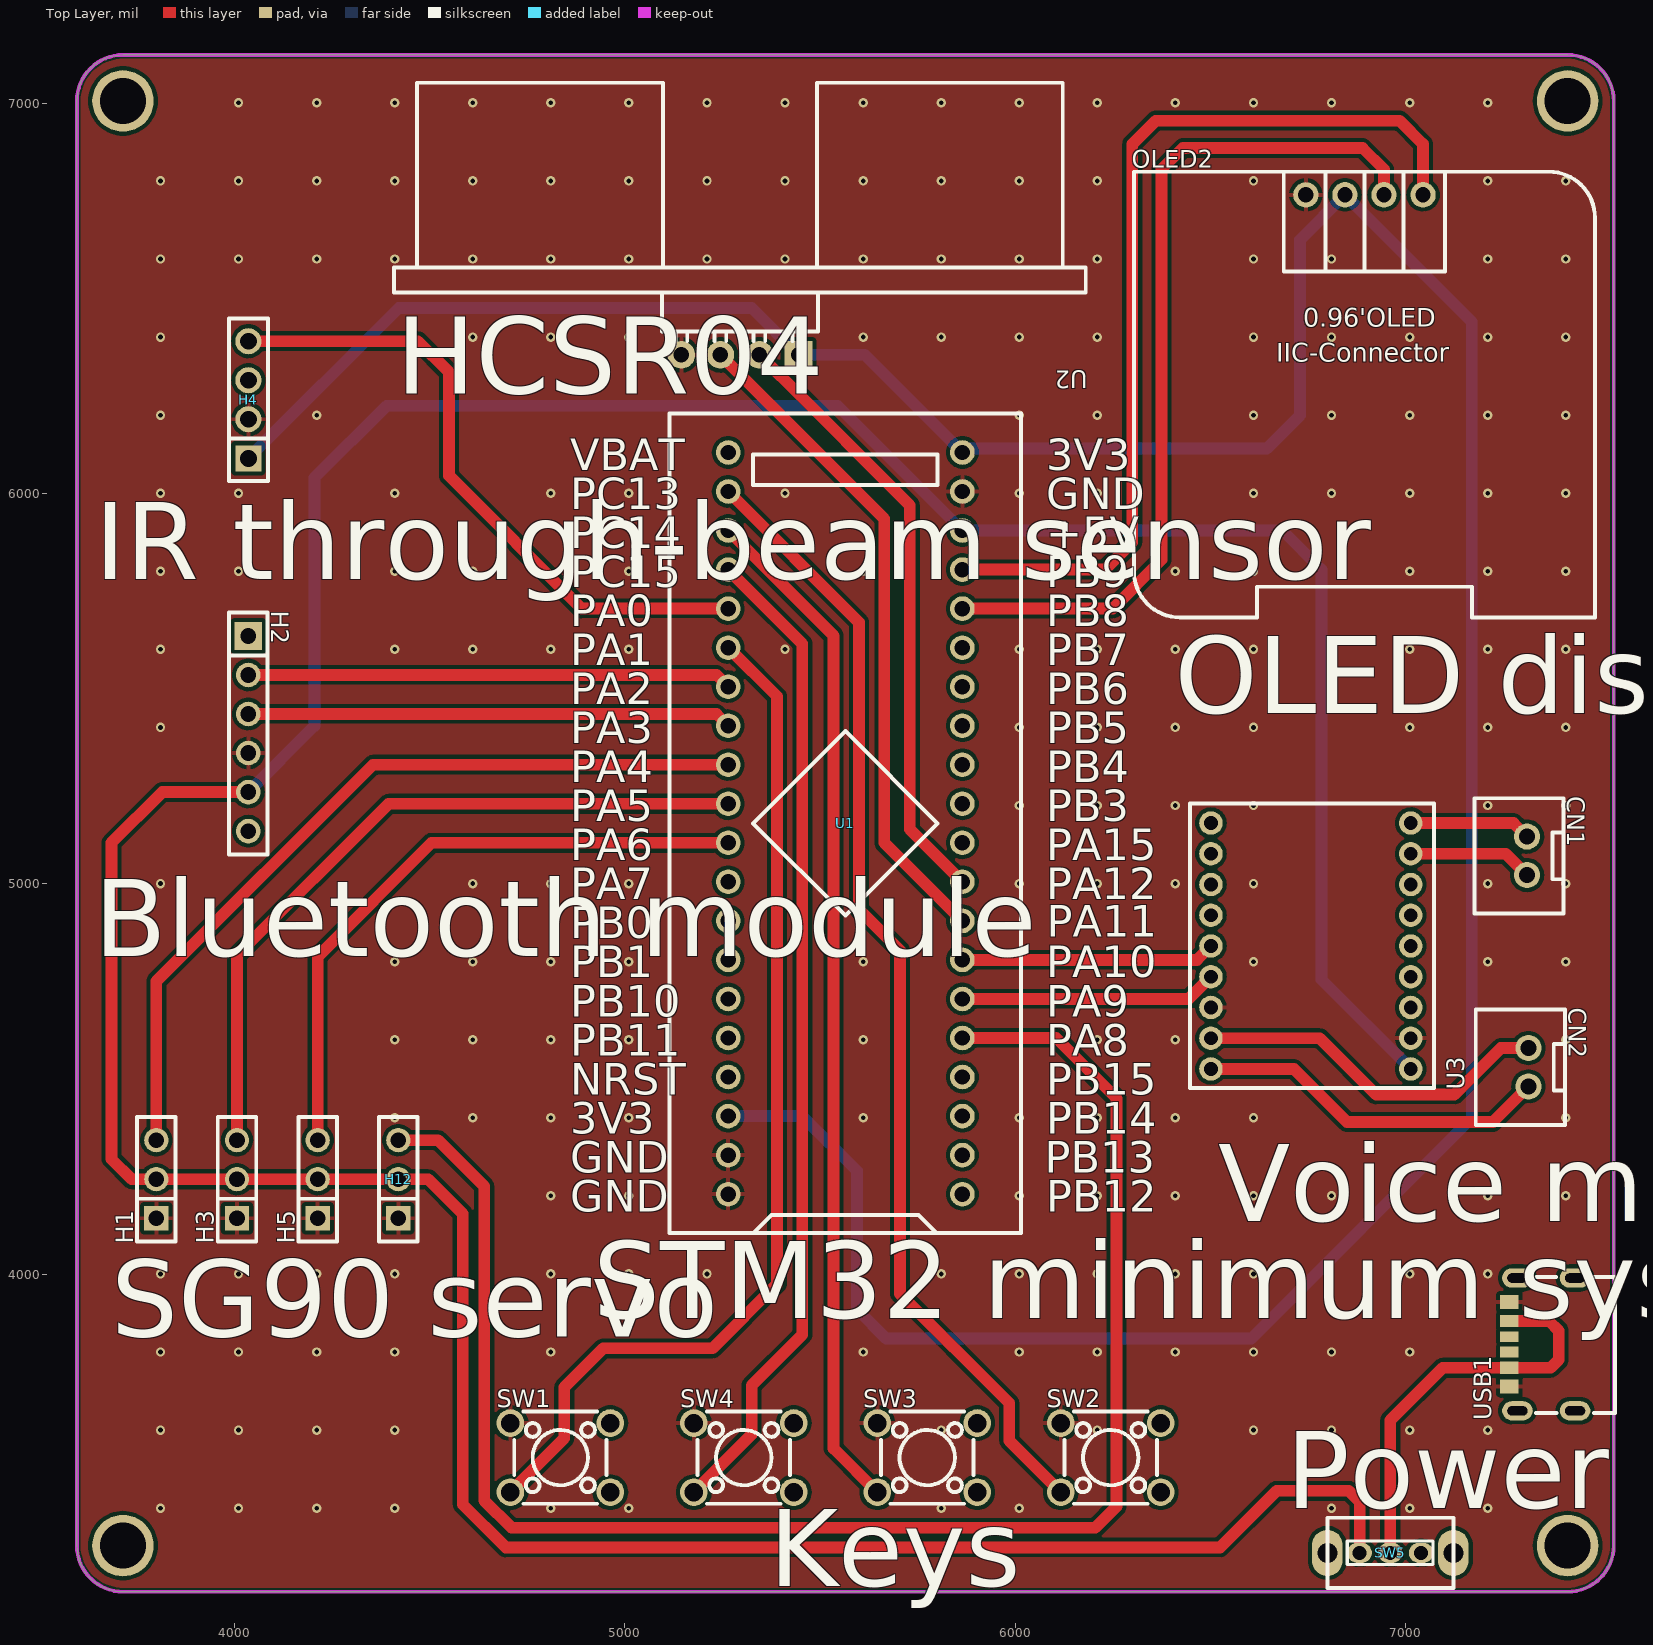
[diagram p0: Top Layer view]
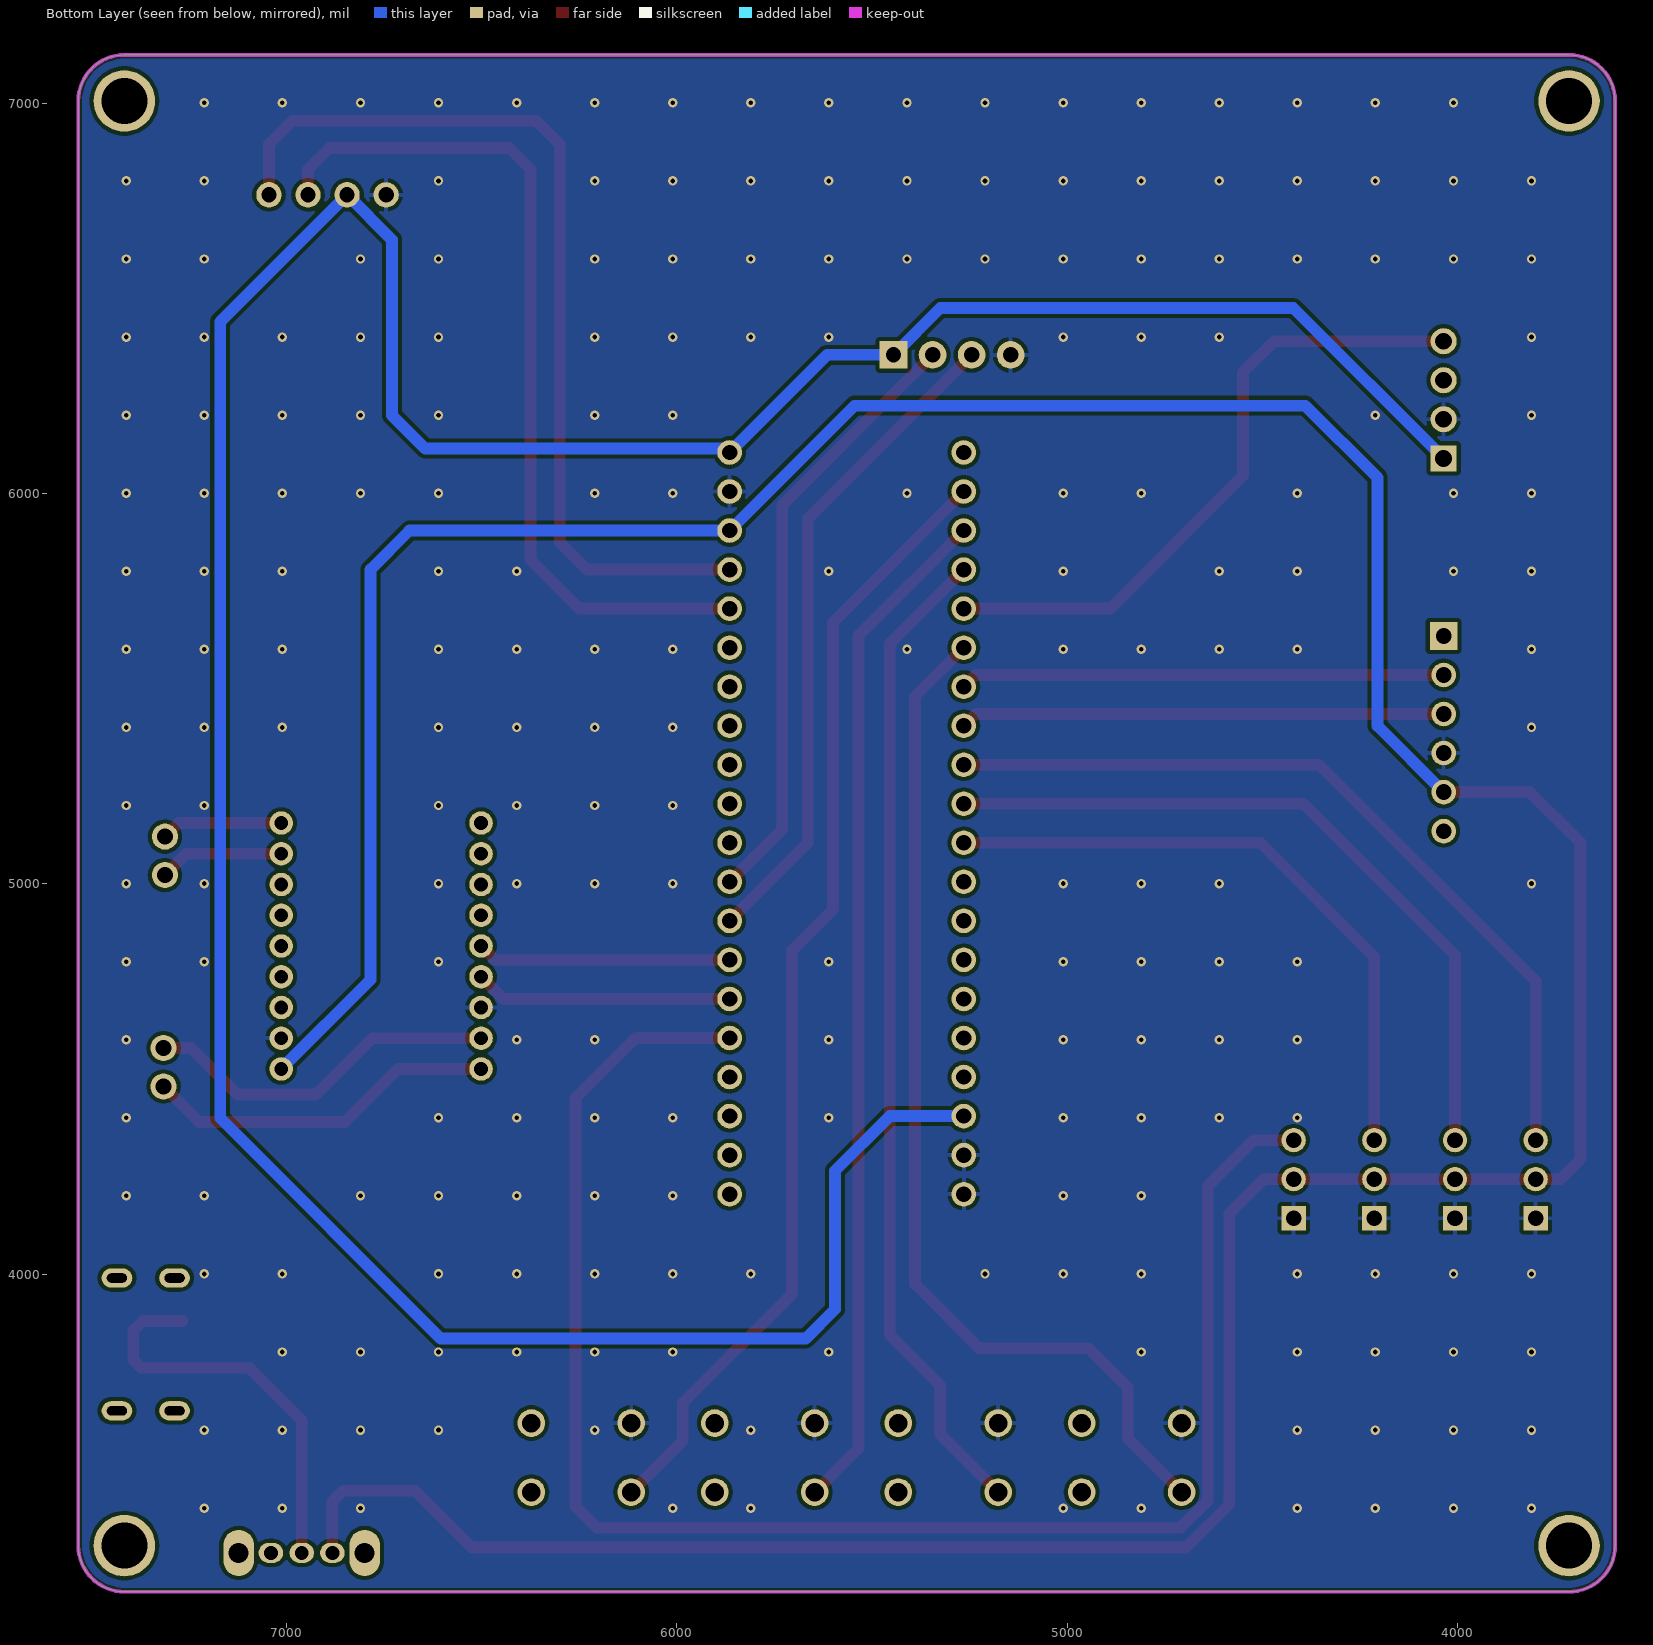
[diagram p1: Bottom Layer view, seen from below]
# Altium PCB MISC51947.pcbdoc
Units mil, origin at the board's own origin, x right, y up, seen from the top; angles counter-clockwise.
Board outline 3937.01 x 3937.01 mil, 2 copper layers (Top Layer, Bottom Layer), stack 62.206 mil thick; 18 components, 42 nets, 127 pads, 215 vias.

## Layer stack, top to bottom
Top Solder Mask Layer: solder mask 0.394, Dk 3.3
Top Layer: signal copper 1.379
Dielectric1: surface 59.449, FR4, Dk 4.5
Bottom Layer: signal copper 1.378
Bottom Solder Mask Layer: solder mask 0.394, Dk 3.3

## Board outline
3714.61,7123.5 ccw(c3714.61,7005.39) 3596.5,7005.39 3596.5,3304.61 ccw(c3714.61,3304.61) 3714.61,3186.5 7415.39,3186.5 ccw(c7415.39,3304.61) 7533.5,3304.61 7533.5,7005.39 ccw(c7415.39,7005.39) 7415.39,7123.5 3714.61,7123.5

## Design rules (kind name [scope] priority, off if disabled: settings)
BoardOutlineClearance copperThickness2oz_1 [All] p2 off: genericclearance=7.99 ignorepadtopadclearanceinfootprint=FALSE except(0: Arc-SplitContinuation Track-SplitContinuation SMDPad-SplitContinuation THPad-SplitContinuation Via-SplitContinuation Fill-SplitContinuation Region-SplitContinuation Poly-SplitContinuation Text-SplitContinuation Hole-SplitContinuation; 5.98: Arc-CutoutEdge Track-CutoutEdge SMDPad-CutoutEdge THPad-CutoutEdge Via-CutoutEdge Text-CutoutEdge; 6.9: Hole-OutlineEdge Hole-CutoutEdge; 10: Poly-OutlineEdge Poly-CutoutEdge; 11.81: Arc-OutlineEdge Track-OutlineEdge SMDPad-OutlineEdge THPad-OutlineEdge Via-OutlineEdge Fill-OutlineEdge Region-OutlineEdge Text-OutlineEdge Fill-CutoutEdge Region-CutoutEdge)
BoardOutlineClearance Plane_innerPlane_1 [All] p4 off: genericclearance=4.02 ignorepadtopadclearanceinfootprint=FALSE except(0: Arc-SplitContinuation Track-SplitContinuation SMDPad-SplitContinuation THPad-SplitContinuation Via-SplitContinuation Fill-SplitContinuation Region-SplitContinuation Poly-SplitContinuation Text-SplitContinuation Hole-SplitContinuation; 5.98: Arc-CutoutEdge Track-CutoutEdge SMDPad-CutoutEdge THPad-CutoutEdge Via-CutoutEdge Text-CutoutEdge; 6.9: Hole-OutlineEdge Hole-CutoutEdge; 10: Poly-OutlineEdge Poly-CutoutEdge; 11.81: Arc-OutlineEdge Track-OutlineEdge SMDPad-OutlineEdge THPad-OutlineEdge Via-OutlineEdge Fill-OutlineEdge Region-OutlineEdge Text-OutlineEdge Fill-CutoutEdge Region-CutoutEdge)
BoardOutlineClearance Copper_copperRegion_1 [All] p6 off: genericclearance=4.02 ignorepadtopadclearanceinfootprint=FALSE except(0: Arc-SplitContinuation Track-SplitContinuation SMDPad-SplitContinuation THPad-SplitContinuation Via-SplitContinuation Fill-SplitContinuation Region-SplitContinuation Poly-SplitContinuation Text-SplitContinuation Hole-SplitContinuation; 5.98: Arc-CutoutEdge Track-CutoutEdge SMDPad-CutoutEdge THPad-CutoutEdge Via-CutoutEdge Text-CutoutEdge; 6.9: Hole-OutlineEdge Hole-CutoutEdge; 10: Poly-OutlineEdge Poly-CutoutEdge; 11.81: Arc-OutlineEdge Track-OutlineEdge SMDPad-OutlineEdge THPad-OutlineEdge Via-OutlineEdge Fill-OutlineEdge Region-OutlineEdge Text-OutlineEdge Fill-CutoutEdge Region-CutoutEdge)
BoardOutlineClearance Copper_copperRegion_copperThickness1oz_1 [All] p8 off: genericclearance=4.02 ignorepadtopadclearanceinfootprint=FALSE except(0: Arc-SplitContinuation Track-SplitContinuation SMDPad-SplitContinuation THPad-SplitContinuation Via-SplitContinuation Fill-SplitContinuation Region-SplitContinuation Poly-SplitContinuation Text-SplitContinuation Hole-SplitContinuation; 5.98: Arc-CutoutEdge Track-CutoutEdge SMDPad-CutoutEdge THPad-CutoutEdge Via-CutoutEdge Text-CutoutEdge; 6.9: Hole-OutlineEdge Hole-CutoutEdge; 10: Poly-OutlineEdge Poly-CutoutEdge; 11.81: Arc-OutlineEdge Track-OutlineEdge SMDPad-OutlineEdge THPad-OutlineEdge Via-OutlineEdge Fill-OutlineEdge Region-OutlineEdge Text-OutlineEdge Fill-CutoutEdge Region-CutoutEdge)
BoardOutlineClearance Copper_copperRegion_Copper_copperRegion_1 [All] p10 off: genericclearance=4.02 ignorepadtopadclearanceinfootprint=FALSE except(0: Arc-SplitContinuation Track-SplitContinuation SMDPad-SplitContinuation THPad-SplitContinuation Via-SplitContinuation Fill-SplitContinuation Region-SplitContinuation Poly-SplitContinuation Text-SplitContinuation Hole-SplitContinuation; 5.98: Arc-CutoutEdge Track-CutoutEdge SMDPad-CutoutEdge THPad-CutoutEdge Via-CutoutEdge Text-CutoutEdge; 6.9: Hole-OutlineEdge Hole-CutoutEdge; 10: Poly-OutlineEdge Poly-CutoutEdge; 11.81: Arc-OutlineEdge Track-OutlineEdge SMDPad-OutlineEdge THPad-OutlineEdge Via-OutlineEdge Fill-OutlineEdge Region-OutlineEdge Text-OutlineEdge Fill-CutoutEdge Region-CutoutEdge)
BoardOutlineClearance copperThickness1oz_1 [All] p12: genericclearance=4.02 ignorepadtopadclearanceinfootprint=FALSE except(0: Arc-SplitContinuation Track-SplitContinuation SMDPad-SplitContinuation THPad-SplitContinuation Via-SplitContinuation Fill-SplitContinuation Region-SplitContinuation Poly-SplitContinuation Text-SplitContinuation Hole-SplitContinuation; 5.98: Arc-CutoutEdge Track-CutoutEdge SMDPad-CutoutEdge THPad-CutoutEdge Via-CutoutEdge Text-CutoutEdge; 6.9: Hole-OutlineEdge Hole-CutoutEdge; 10: Poly-OutlineEdge Poly-CutoutEdge; 11.81: Arc-OutlineEdge Track-OutlineEdge SMDPad-OutlineEdge THPad-OutlineEdge Via-OutlineEdge Fill-OutlineEdge Region-OutlineEdge Text-OutlineEdge Fill-CutoutEdge Region-CutoutEdge)
Clearance copperThickness2oz [All] p1 off: gap=7.99 ignorepadtopadclearanceinfootprint=FALSE except(5.98: SMDPad-Track SMDPad-SMDPad THPad-Track SMDPad-THPad THPad-THPad Track-Via SMDPad-Via THPad-Via Via-Via Fill-SMDPad Region-SMDPad Fill-THPad Region-THPad Fill-Via Region-Via Fill-Fill Fill-Region Region-Region Arc-Track Arc-SMDPad Arc-THPad Arc-Via Fill-Arc Region-Arc Arc-Arc Text-Track SMDPad-Text Text-THPad Text-Via Fill-Text Region-Text Arc-Text Text-Text; 6.9: Hole-Track Hole-SMDPad Hole-THPad Hole-Via Fill-Hole Region-Hole Hole-Arc Hole-Text; 10: Poly-Track Poly-SMDPad Poly-THPad Poly-Via Poly-Fill Poly-Region Poly-Poly Poly-Arc Poly-Text Poly-Hole; 11.81: Fill-Track Region-Track)
Clearance Plane_innerPlane [All] p3 off: gap=4.02 ignorepadtopadclearanceinfootprint=FALSE except(5.98: SMDPad-Track SMDPad-SMDPad THPad-Track SMDPad-THPad THPad-THPad Track-Via SMDPad-Via THPad-Via Via-Via Fill-SMDPad Region-SMDPad Fill-THPad Region-THPad Fill-Via Region-Via Fill-Fill Fill-Region Region-Region Arc-Track Arc-SMDPad Arc-THPad Arc-Via Fill-Arc Region-Arc Arc-Arc Text-Track SMDPad-Text Text-THPad Text-Via Fill-Text Region-Text Arc-Text Text-Text; 6.9: Hole-Track Hole-SMDPad Hole-THPad Hole-Via Fill-Hole Region-Hole Hole-Arc Hole-Text; 10: Poly-Track Poly-SMDPad Poly-THPad Poly-Via Poly-Fill Poly-Region Poly-Poly Poly-Arc Poly-Text Poly-Hole; 11.81: Fill-Track Region-Track)
Clearance Copper_copperRegion [All] p5 off: gap=4.02 ignorepadtopadclearanceinfootprint=FALSE except(5.98: SMDPad-Track SMDPad-SMDPad THPad-Track SMDPad-THPad THPad-THPad Track-Via SMDPad-Via THPad-Via Via-Via Fill-SMDPad Region-SMDPad Fill-THPad Region-THPad Fill-Via Region-Via Fill-Fill Fill-Region Region-Region Arc-Track Arc-SMDPad Arc-THPad Arc-Via Fill-Arc Region-Arc Arc-Arc Text-Track SMDPad-Text Text-THPad Text-Via Fill-Text Region-Text Arc-Text Text-Text; 6.9: Hole-Track Hole-SMDPad Hole-THPad Hole-Via Fill-Hole Region-Hole Hole-Arc Hole-Text; 10: Poly-Track Poly-SMDPad Poly-THPad Poly-Via Poly-Fill Poly-Region Poly-Poly Poly-Arc Poly-Text Poly-Hole; 11.81: Fill-Track Region-Track)
Clearance Copper_copperRegion_copperThickness1oz [All] p7 off: gap=4.02 ignorepadtopadclearanceinfootprint=FALSE except(5.98: SMDPad-Track SMDPad-SMDPad THPad-Track SMDPad-THPad THPad-THPad Track-Via SMDPad-Via THPad-Via Via-Via Fill-SMDPad Region-SMDPad Fill-THPad Region-THPad Fill-Via Region-Via Fill-Fill Fill-Region Region-Region Arc-Track Arc-SMDPad Arc-THPad Arc-Via Fill-Arc Region-Arc Arc-Arc Text-Track SMDPad-Text Text-THPad Text-Via Fill-Text Region-Text Arc-Text Text-Text; 6.9: Hole-Track Hole-SMDPad Hole-THPad Hole-Via Fill-Hole Region-Hole Hole-Arc Hole-Text; 10: Poly-Track Poly-SMDPad Poly-THPad Poly-Via Poly-Fill Poly-Region Poly-Poly Poly-Arc Poly-Text Poly-Hole; 11.81: Fill-Track Region-Track)
Clearance Copper_copperRegion_Copper_copperRegion [All] p9 off: gap=4.02 ignorepadtopadclearanceinfootprint=FALSE except(5.98: SMDPad-Track SMDPad-SMDPad THPad-Track SMDPad-THPad THPad-THPad Track-Via SMDPad-Via THPad-Via Via-Via Fill-SMDPad Region-SMDPad Fill-THPad Region-THPad Fill-Via Region-Via Fill-Fill Fill-Region Region-Region Arc-Track Arc-SMDPad Arc-THPad Arc-Via Fill-Arc Region-Arc Arc-Arc Text-Track SMDPad-Text Text-THPad Text-Via Fill-Text Region-Text Arc-Text Text-Text; 6.9: Hole-Track Hole-SMDPad Hole-THPad Hole-Via Fill-Hole Region-Hole Hole-Arc Hole-Text; 10: Poly-Track Poly-SMDPad Poly-THPad Poly-Via Poly-Fill Poly-Region Poly-Poly Poly-Arc Poly-Text Poly-Hole; 11.81: Fill-Track Region-Track)
Clearance copperThickness1oz [All] p11: gap=4.02 ignorepadtopadclearanceinfootprint=FALSE except(5.98: SMDPad-Track SMDPad-SMDPad THPad-Track SMDPad-THPad THPad-THPad Track-Via SMDPad-Via THPad-Via Via-Via Fill-SMDPad Region-SMDPad Fill-THPad Region-THPad Fill-Via Region-Via Fill-Fill Fill-Region Region-Region Arc-Track Arc-SMDPad Arc-THPad Arc-Via Fill-Arc Region-Arc Arc-Arc Text-Track SMDPad-Text Text-THPad Text-Via Fill-Text Region-Text Arc-Text Text-Text; 6.9: Hole-Track Hole-SMDPad Hole-THPad Hole-Via Fill-Hole Region-Hole Hole-Arc Hole-Text; 10: Poly-Track Poly-SMDPad Poly-THPad Poly-Via Poly-Fill Poly-Region Poly-Poly Poly-Arc Poly-Text Poly-Hole; 11.81: Fill-Track Region-Track)
DiffPairsRouting differentialPair [All] p1: maxlimit=6 minlimit=6 mostfreqgap=6 toplayer_minwidth=5 toplayer_prefwidth=10 toplayer_maxwidth=100 toplayer_mingap=6 toplayer_prefgap=6 toplayer_maxgap=6 bottomlayer_minwidth=5 bottomlayer_prefwidth=10 bottomlayer_maxwidth=100 bottomlayer_mingap=6 bottomlayer_prefgap=6 bottomlayer_maxgap=6 maxuncoupledlength=10
HoleToHoleClearance otherClearance [All] p1: gap=11.81 allowstackedmicrovias=TRUE
Length netLength [All] p1: minlimit=0 maxlimit=0
PasteMaskExpansion pasteMaskExpansion [All] p1: expansion=0
PlaneConnect innerPlane [All] p1: planeconnectstyle=Relief reliefexpansion=20 reliefentries=4 reliefconductorwidth=10 reliefairgap=10
PolygonConnect copperRegion_copperThickness1oz [All] p1 off: connectstyle=Relief reliefconductorwidth=10 reliefentries=4 polygonreliefangle="90 Angle" airgapwidth=10 via.connectstyle=Relief via.reliefconductorwidth=10 via.reliefentries=4 via.polygonreliefangle="90 Angle" via.airgapwidth=10
PolygonConnect copperRegion_Copper_copperRegion [All] p2 off: connectstyle=Relief reliefconductorwidth=10 reliefentries=4 polygonreliefangle="90 Angle" airgapwidth=10 via.connectstyle=Relief via.reliefconductorwidth=10 via.reliefentries=4 via.polygonreliefangle="90 Angle" via.airgapwidth=10
PolygonConnect copperRegion [All] p3: connectstyle=Relief reliefconductorwidth=10 reliefentries=4 polygonreliefangle="90 Angle" airgapwidth=10 via.connectstyle=Relief via.reliefconductorwidth=10 via.reliefentries=4 via.polygonreliefangle="90 Angle" via.airgapwidth=10
RoutingVias viaSize [All] p1: holewidth=12.01 width=24.02 viastyle="Through Hole" minholewidth=11.81 minwidth=19.68 maxholewidth=248.03 maxwidth=393.7
SolderMaskExpansion solderMaskExpansion [IsVia] p1: expansion=-1000 istentingtop=TRUE
SolderMaskExpansion solderMaskExpansion [All] p2: expansion=2 istentingtop=FALSE
Width copperThickness2oz_2 [All] p1 off: maxlimit=100 minlimit=8 preferedwidth=10
Width copperThickness1oz_2 [All] p2: maxlimit=100 minlimit=5 preferedwidth=10

## Components (designator, comment, footprint, x,y, rotation, side; value= is the part's Value field where it differs from the comment)
CN1 "XH2.54*2P_THT" CONN-TH_2P-P2.50-XH2.54-2P 7311.56,5071.57 r270 top
CN2 "XH2.54*2P_THT" CONN-TH_2P-P2.50-XH2.54-2P 7315,4530 r270 top
H1 "" HDR-TH_3P-P2.54-V-F 3800,4243.21 r90 top
H2 "" HDR-TH_6P-P2.54-V-F 4035.79,5385 r270 top
H3 "" HDR-TH_3P-P2.54-V-F 4006.67,4243.21 r90 top
H4 "" HDR-TH_4P-P2.54-V-F 4035.79,6240 r90 top
H5 "" HDR-TH_3P-P2.54-V-F 4213.33,4243.21 r90 top
H12 "" HDR-TH_3P-P2.54-V-F 4420,4243.21 r90 top
OLED2 "" 0.96OLED_4P 6895,6765 r0 top
SW1 "" SW-TH_4P-L6.0-W6.0-P4.50-LS6.5 4835,3530 r0 top
SW2 "" SW-TH_4P-L6.0-W6.0-P4.50-LS6.5 6245,3530 r0 top
SW3 "" SW-TH_4P-L6.0-W6.0-P4.50-LS6.5 5775,3530 r0 top
SW4 "" SW-TH_4P-L6.0-W6.0-P4.50-LS6.5 5305,3530 r0 top
SW5 "" 拨动开关 6956,3286 r0 top
U1 "STM32F103C8T6-Card" CONN-TH_L53.3-W22.9_STM32F103C8T6-CARD 5565,5155 r90 top
U2 "HC-SR04" TH_HC-SR04V 5295,6355 r180 top
U3 "CON2.0MM-PAD-18" CONN-TH_18P-P2.00_C9900078766 7013.53,4840.71 r90 top
USB1 "" "USB_ TYPE-C-6P" 7350.24,3815.09 r90 top

## Footprints (in the part's own frame and the unit in brackets; to place one, negate y for a bottom-side part, rotate by r counter-clockwise, add the part's x,y. Pads: shape width x height; smd on the part's side, far side on the other; paste and mask are expansions set on the pad)
0.96OLED_4P [mm]
  round 1.65 hole 1 copper offset 0,0: 1(-3.81,-0.001) 2(-1.27,0.002) 3(1.27,0.002) 4(3.81,0.002)
  silkscreen extent -15,-27.5 15,1.5
CONN-TH_2P-P2.50-XH2.54-2P [mm]
  round 1.7 hole 1.05 paste+0 mask+0.05: 1(1.25,0) 2(-1.25,0)
  silkscreen extent -3.75,-3.42 3.75,2.37
CONN-TH_18P-P2.00_C9900078766 [mil]
  round 60 hole 35.43 paste+0 mask+1.97: 1(-314.96,0.01) 2(-314.96,511.81) 3(-236.22,0.01) 4(-236.22,511.81) 5(-157.48,0.01) 6(-157.48,511.81) 9(0,0) 10(0,511.81) 11(78.74,0) 12(78.74,511.81) 13(157.48,0) 14(157.48,511.81) 15(236.22,0) 16(236.22,511.81) 17(314.96,0) 18(314.96,511.81)
  round 60 hole 35.43 copper offset -0.01,0 paste+0 mask+1.97: 7(-78.72,0.01) 8(-78.72,511.81)
  silkscreen extent -363,-60 365,565
CONN-TH_L53.3-W22.9_STM32F103C8T6-CARD [mm]
  round 1.6 hole 1: 1(-24.13,-7.62) 2(-21.59,-7.62) 3(-19.05,-7.62) 4(-16.51,-7.62) 5(-13.97,-7.62) 6(-11.43,-7.62) 7(-8.89,-7.62) 8(-6.35,-7.62) 9(-3.81,-7.62) 10(-1.27,-7.62) 11(1.27,-7.62) 12(3.81,-7.62) 13(6.35,-7.62) 14(8.89,-7.62) 15(11.43,-7.62) 16(13.97,-7.62) 17(16.51,-7.62) 18(19.05,-7.62) 19(21.59,-7.62) 20(24.13,-7.62) 21(24.13,7.62) 22(21.59,7.62) 23(19.05,7.62) 24(16.51,7.62) 25(13.97,7.62) 26(11.43,7.62) 27(8.89,7.62) 28(6.35,7.62) 29(3.81,7.62) 30(1.27,7.62) 31(-1.27,7.62) 32(-3.81,7.62) 33(-6.35,7.62) 34(-8.89,7.62) 35(-11.43,7.62) 36(-13.97,7.62) 37(-16.51,7.62) 38(-19.05,7.62) 39(-21.59,7.62) 40(-24.13,7.62)
  silkscreen extent -26.67,-11.43 26.67,11.43
HDR-TH_3P-P2.54-V-F [mil]
  rect 62x62 hole 40.16: 1(-100,0)
  round 62 hole 40.16: 2(0,0) 3(100,0)
  silkscreen extent -160,-49 160,49
HDR-TH_4P-P2.54-V-F [mm]
  rect 1.7x1.7 hole 1.1: 1(-3.81,0)
  round 1.7 hole 1.1: 2(-1.27,0) 3(1.27,0) 4(3.81,0)
  silkscreen extent -5.29,-1.27 5.29,1.27
HDR-TH_6P-P2.54-V-F [mm]
  rect 1.8x1.8 hole 1.02: 1(-6.35,0)
  round 1.6 hole 1.02: 2(-3.81,0) 3(-1.27,0) 4(1.27,0) 5(3.81,0) 6(6.35,0)
  silkscreen extent -7.87,-1.25 7.87,1.25
SW-TH_4P-L6.0-W6.0-P4.50-LS6.5 [mm]
  round 1.8 hole 1.2: 1(-3.25,2.25) 2(3.25,2.25) 3(-3.25,-2.25) 4(3.25,-2.25)
  silkscreen extent -3,-3 3,3
TH_HC-SR04V [mm]
  rect 1.8x1.8 hole 1.001: 1(-3.81,0)
  round 1.8 hole 1.001: 2(-1.27,0) 3(1.27,0) 4(3.81,0)
  silkscreen extent -22.5,-17.7 22.5,-0.89
"USB_ TYPE-C-6P" [mm]
  oval 1.25x2 hole 0.6 slot 1.3 at 90 deg paste+0 mask+0.05: 7(-4.193,1.611) 8(4.447,1.611) 9(-4.193,-2.139) 10(4.447,-2.139)
  rect 0.7x1.2 smd paste-100 mask+0.05: A5(-0.373,2.139) B5(0.627,2.139)
  rect 0.8x1.2 smd paste-100 mask+0.05: A9(1.647,2.139) B9(-1.393,2.139)
  rect 0.9x1.2 smd paste-100 mask+0.05: A12(2.877,2.139) B12(-2.623,2.139)
  silkscreen extent -4.34,-4.75 4.52,0.39
拨动开关 [mil]
  oval 63x51.2 hole 35.4 paste+0 mask+2: 1(-73.4,0) 2(5,0) 3(84,0)
  oval 78.7x118.1 hole 51.2 paste+0 mask+2: 4(166.7,0) 5(-156.1,0)
  silkscreen extent -156,-90 167,90

## Free pads (board coordinates)
  round 157.48 hole 118.11: 1(3714.61,7005.39) 1(3714.61,3304.61) 1(7415.39,7005.39) 1(7415.39,3304.61)

## Via types
v1: diameter 24.02, hole 12, Top Layer to Bottom Layer, 215 vias

## Nets (pads, with @x,y where several pads share a name; then routed paths per layer and width w, separated by ;. In a path a pad name is that pad's centre, name@x,y a point inside that pad or via, vN(x,y) a via of type N, cw(c..) or ccw(c..) an arc to the next point about the centre after c; other vN are vias at no path point)
$1N17172: SW5.2 USB1.A9 USB1.B9 | length 1046.6
  Top Layer w30: SW5.2 6961,3626 7095.25,3760.25 USB1.B9 7371.97,3760.25 7392.43,3780.7 7392.43,3855.17 7367.68,3879.93 USB1.A9
+5V: H1.2 H2.5 H3.2 H5.2 H12.2 SW5.1 U1.18 U3.1 | length 10543.3
  Top Layer w30: H2.5 3815,5235 3685,5105 3685,4295 3736.79,4243.21 H1.2 H3.2 H5.2 H12.2 4496.79,4243.21 4585,4155 4585,3410 4695,3300 6525,3300 6670,3445 6855,3445 6882.6,3417.4 SW5.1
  Bottom Layer w30: H2.5 4205,5404.21 4205,6040 4390,6225 5545,6225 U1.18 6685,5905 6785,5805 6785,4754.27 U3.1
GND: H1.1 H2.4 H3.1 H4.2 H5.1 H12.1 OLED2.1 SW1.1 SW2.1 SW3.1 SW4.1 U1.19 U1.39 U1.40 U2.4 U3.3 U3.6 USB1.A12 USB1.B12
  other v1: 3810.6,3400.6 4010.6,3400.6 4210.6,3400.6 4410.6,3400.6 4810.6,3400.6 5010.6,3400.6 5810.6,3400.6 6010.6,3400.6 6810.6,3400.6 7010.6,3400.6 7210.6,3400.6 3810.6,3600.6 4010.6,3600.6 4210.6,3600.6 4410.6,3600.6 5810.6,3600.6 6210.6,3600.6 6610.6,3600.6 6810.6,3600.6 7010.6,3600.6 7210.6,3600.6 3810.6,3800.6 4010.6,3800.6 4210.6,3800.6 4410.6,3800.6 4810.6,3800.6 5610.6,3800.6 6010.6,3800.6 6210.6,3800.6 6410.6,3800.6 6610.6,3800.6 6810.6,3800.6 7010.6,3800.6 3810.6,4000.6 4010.6,4000.6 4210.6,4000.6 4410.6,4000.6 4810.6,4000.6 5010.6,4000.6 5210.6,4000.6 5810.6,4000.6 6010.6,4000.6 6210.6,4000.6 6410.6,4000.6 6610.6,4000.6 7010.6,4000.6 7210.6,4000.6 4810.6,4200.6 5010.6,4200.6 6010.6,4200.6 6210.6,4200.6 6410.6,4200.6 6610.6,4200.6 6810.6,4200.6 7210.6,4200.6 7410.6,4200.6 4410.6,4400.6 4610.6,4400.6 4810.6,4400.6 5010.6,4400.6 5610.6,4400.6 6010.6,4400.6 6210.6,4400.6 6410.6,4400.6 6610.6,4400.6 7410.6,4400.6 4410.6,4600.6 4610.6,4600.6 4810.6,4600.6 5010.6,4600.6 5610.6,4600.6 6210.6,4600.6 6410.6,4600.6 7410.6,4600.6 4410.6,4800.6 4610.6,4800.6 4810.6,4800.6 5010.6,4800.6 5610.6,4800.6 6610.6,4800.6 7210.6,4800.6 7410.6,4800.6 3810.6,5000.6 4610.6,5000.6 4810.6,5000.6 5010.6,5000.6 6010.6,5000.6 6210.6,5000.6 6410.6,5000.6 6610.6,5000.6 7210.6,5000.6 7410.6,5000.6 6010.6,5200.6 6210.6,5200.6 6410.6,5200.6 6610.6,5200.6 7210.6,5200.6 7410.6,5200.6 3810.6,5400.6 6010.6,5400.6 6210.6,5400.6 6410.6,5400.6 6610.6,5400.6 7010.6,5400.6 7210.6,5400.6 7410.6,5400.6 3810.6,5600.6 4410.6,5600.6 4610.6,5600.6 4810.6,5600.6 5010.6,5600.6 5410.6,5600.6 6010.6,5600.6 6210.6,5600.6 6410.6,5600.6 6610.6,5600.6 7010.6,5600.6 7210.6,5600.6 7410.6,5600.6 3810.6,5800.6 4010.6,5800.6 4410.6,5800.6 4610.6,5800.6 5010.6,5800.6 5610.6,5800.6 6410.6,5800.6 6610.6,5800.6 7010.6,5800.6 7210.6,5800.6 7410.6,5800.6 3810.6,6000.6 4010.6,6000.6 4410.6,6000.6 4810.6,6000.6 5010.6,6000.6 5410.6,6000.6 6010.6,6000.6 6210.6,6000.6 6610.6,6000.6 6810.6,6000.6 7010.6,6000.6 7210.6,6000.6 7410.6,6000.6 3810.6,6200.6 4210.6,6200.6 6010.6,6200.6 6210.6,6200.6 6610.6,6200.6 6810.6,6200.6 7010.6,6200.6 7210.6,6200.6 7410.6,6200.6 3810.6,6400.6 4610.6,6400.6 4810.6,6400.6 5010.6,6400.6 5610.6,6400.6 5810.6,6400.6 6010.6,6400.6 6210.6,6400.6 6610.6,6400.6 6810.6,6400.6 7010.6,6400.6 7210.6,6400.6 7410.6,6400.6 3810.6,6600.6 4010.6,6600.6 4210.6,6600.6 4410.6,6600.6 4610.6,6600.6 4810.6,6600.6 5010.6,6600.6 5210.6,6600.6 5410.6,6600.6 5610.6,6600.6 5810.6,6600.6 6010.6,6600.6 6210.6,6600.6 6610.6,6600.6 6810.6,6600.6 7210.6,6600.6 7410.6,6600.6 3810.6,6800.6 4010.6,6800.6 4210.6,6800.6 4410.6,6800.6 4610.6,6800.6 4810.6,6800.6 5010.6,6800.6 5210.6,6800.6 5410.6,6800.6 5610.6,6800.6 5810.6,6800.6 6010.6,6800.6 6210.6,6800.6 6610.6,6800.6 7210.6,6800.6 7410.6,6800.6 4010.6,7000.6 4210.6,7000.6 4410.6,7000.6 4610.6,7000.6 4810.6,7000.6 5010.6,7000.6 5210.6,7000.6 5410.6,7000.6 5610.6,7000.6 5810.6,7000.6 6010.6,7000.6 6210.6,7000.6 6410.6,7000.6 6610.6,7000.6 6810.6,7000.6 7010.6,7000.6 7210.6,7000.6
MIC+: CN1.1 U3.15 | length 320.6
  Top Layer w30: U3.15 7256.99,5076.93 CN1.1
MIC-: CN1.2 U3.17 | length 312.5
  Top Layer w30: U3.17 7276.68,5155.67 CN1.2
NRST: U1.37
PA0: H4.4 U1.25 | length 1668.2
  Top Layer w30: H4.4 4470,6390 4550,6310 4550,6045 4890,5705 U1.25
PA1: SW1.3 U1.26 | length 2662.3
  Top Layer w30: SW1.3 4845,3579.37 4845,3710 4945,3810 5225,3810 5390,3975 5390,5480 U1.26
PA2: H2.2 U1.27 | length 1241.6
  Top Layer w30: H2.2 5235,5535 U1.27
PA3: H2.3 U1.28 | length 1241.6
  Top Layer w30: H2.3 5235,5435 U1.28
PA4: H1.3 U1.29 | length 2101.7
  Top Layer w30: H1.3 3800,4750 4355,5305 U1.29
PA5: H3.3 U1.30 | length 1892.6
  Top Layer w30: H3.3 4006.67,4816.67 4395,5205 U1.30
PA6: H5.3 U1.31 | length 1642.6
  Top Layer w30: H5.3 4213.33,4813.33 4505,5105 U1.31
PA7: U1.32
PA8: H12.3 U1.5 | length 4249.9
  Top Layer w30: H12.3 4521.79,4343.21 4640,4225 4640,3420 4710,3350 6205,3350 6260,3405 6260,4450 6105,4605 U1.5
PA9: U1.6 U3.8 | length 660.3
  Top Layer w30: U1.6 6444.75,4705 U3.8
PA10: U1.7 U3.10 | length 651.5
  Top Layer w30: U1.7 6466.02,4805 U3.10
PA11: U1.8 U2.3 | length 1706.8
  Top Layer w30: U2.3 5665,5935 5665,5105 U1.8
PA12: U1.9 U2.2 | length 1565.4
  Top Layer w30: U2.2 5392.18,6307.82 ccw(c5409.57,6319.57) 5397.82,6302.18 5730,5970 5730,5140 U1.9
PA15: U1.10
PB0: U1.33
PB1: U1.34
PB3: U1.11
PB4: U1.12
PB5: U1.13
PB6: U1.14
PB7: U1.15
PB8: OLED2.3 U1.16 | length 2242.3
  Top Layer w30: U1.16 6250,5705 6375,5830 6375,6830 6430,6885 6890,6885 6945,6830 OLED2.3@6945,6765.05
PB9: OLED2.4 U1.17 | length 2408.7
  Top Layer w30: U1.17 6230,5805 6300,5875 6300,6895 6360,6955 6985,6955 7045,6895 OLED2.4@7045,6765.05
PB10: U1.35
PB11: U1.36
PB12: U1.1
PB13: U1.2
PB14: U1.3
PB15: U1.4
PC13: SW2.3 U1.22 | length 2916.5
  Top Layer w30: U1.22 5600,5670 5600,4935 5705,4830 5705,3950 5985,3670 5985,3573.47 SW2.3
PC14: SW3.3 U1.23 | length 2621.8
  Top Layer w30: U1.23 5535,5635 5535,3553.47 SW3.3
PC15: SW4.3 U1.24 | length 2557.4
  Top Layer w30: SW4.3 5325,3589.37 5325,3715 5455,3845 5455,5615 U1.24
SPK+: CN2.1 U3.2 | length 907.1
  Top Layer w30: U3.2 6714.25,4525.75 6850,4390 7224.22,4390 CN2.1
SPK-: CN2.2 U3.4 | length 922.5
  Top Layer w30: U3.4 6780.51,4604.49 6925,4460 7125,4460 7244.22,4579.22 CN2.2
VBAT: U1.21
VCC: H4.1 OLED2.2 U1.20 U1.38 U2.1 | length 8741.7
  Bottom Layer w30: H4.1 4420.79,6475 5325,6475 U2.1 5615,6355 U1.20 5875,6115 6645,6115 6730,6200 6730,6650.05 6845,6765.05 7170,6440.05 7170,4400 6605,3835 5670,3835 5595,3910 5595,4265 5455,4405 U1.38
pads on no net: H2.1 H2.6 H4.3 SW1.2 SW1.4 SW2.2 SW2.4 SW3.2 SW3.4 SW4.2 SW4.4 SW5.3 SW5.4 SW5.5 U3.5 U3.7 U3.9 U3.11 U3.12 U3.13 U3.14 U3.16 U3.18 USB1.7 USB1.8 USB1.9 USB1.10 USB1.A5 USB1.B5

## Polygon pours and split planes (outlines as drawn)
GND on Bottom Layer (solid, remove dead copper, pour order 2): 3525,7245 3525,3080 7700,3080 7700,7245
GND on Top Layer (solid, remove dead copper, pour order 2): 3000,7415 3000,3000 7930,3000 7930,7415

## Keep-outs
Board Outline Layer:
  the board outline again, w10

## Silkscreen, mask and mechanical layers (free items; w line width, h text height)
Top Silkscreen Layer:
  text "HCSR04" at 4415,6255 h196.85
  text "VBAT" at 4860.95,6060 h80
  text "3V3" at 6079.16,6060 h80
  text "PC13" at 4860.95,5960 h80
  text "GND" at 6079.16,5960 h80
  text "PC14" at 4860.95,5860 h80
  text "+5V" at 6079.16,5860 h80
  text "IR through-beam sensor" at 3642.39,5780 h196.85
  text "PC15" at 4860.95,5760 h80
  text "PB9" at 6079.16,5760 h80
  text "PA0" at 4860.95,5660 h80
  text "PB8" at 6079.16,5660 h80
  text "PA1" at 4860.95,5560 h80
  text "PB7" at 6079.16,5560 h80
  text "PA2" at 4860.95,5460 h80
  text "PB6" at 6079.16,5460 h80
  text "OLED display" at 6408.66,5436.57 h196.85
  text "PA3" at 4860.95,5360 h80
  text "PB5" at 6079.16,5360 h80
  text "PA4" at 4860.95,5260 h80
  text "PB4" at 6079.16,5260 h80
  text "PA5" at 4860.95,5160 h80
  text "PB3" at 6079.16,5160 h80
  text "PA6" at 4860.95,5060 h80
  text "PA15" at 6079.16,5060 h80
  text "PA7" at 4860.95,4960 h80
  text "PA12" at 6079.16,4960 h80
  text "PA11" at 6080.95,4865 h80
  text "PB0" at 4860.95,4860 h80
  text "Bluetooth module" at 3641.38,4815 h196.85
  text "PB1" at 4860.95,4760 h80
  text "PA10" at 6079.16,4760 h80
  text "PB10" at 4860.95,4660 h80
  text "PA9" at 6079.16,4660 h80
  text "PB11" at 4860.95,4560 h80
  text "PA8" at 6079.16,4560 h80
  text "NRST" at 4860.95,4460 h80
  text "PB15" at 6079.16,4460 h80
  text "3V3" at 4860.95,4360 h80
  text "PB14" at 6079.16,4360 h80
  text "GND" at 4860.95,4260 h80
  text "PB13" at 6075.95,4260 h80
  text "GND" at 4860.95,4160 h80
  text "PB12" at 6079.16,4160 h80
  text "Voice module" at 6520,4135 h196.85
  text "STM32 minimum system" at 4919.45,3886.57 h196.85
  text "SG90 servo" at 3685,3840 h196.85
  text "Power connector" at 6695,3400 h196.85
  text "Keys" at 5370,3200 h196.85